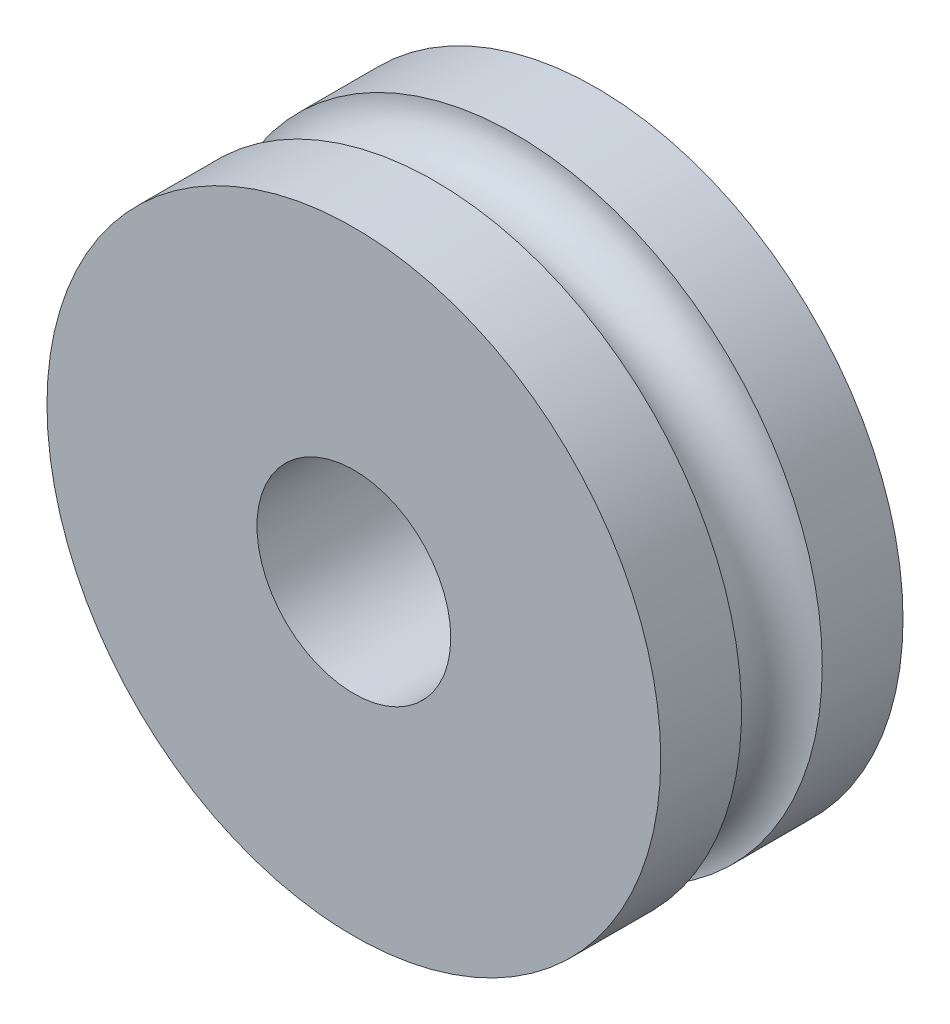
from build123d import *

# Parameters (mm, degrees)
SKETCH1_R           = 38
SKETCH1_R_2         = 12
BOSS_EXTRUDE1_DEPTH = 30
SKETCH2_R           = 5


with BuildPart() as part:
    # Sketch1 → Boss-Extrude1 (new body)
    with BuildSketch(Plane.XY):
        Circle(SKETCH1_R)
        Circle(SKETCH1_R_2, mode=Mode.SUBTRACT)
    extrude(amount=BOSS_EXTRUDE1_DEPTH)

    # Sketch2 → Cut-Revolve1 (revolve, cut)
    with BuildSketch(Plane(origin=(0, 0, 0), x_dir=(1, 0, 0), z_dir=(0, 1, 0))):
        with Locations((-38, -15)):
            Circle(SKETCH2_R)
    revolve(axis=Axis((0, 0, 0), (0, 0, 1)), mode=Mode.SUBTRACT)


solid = part.part
